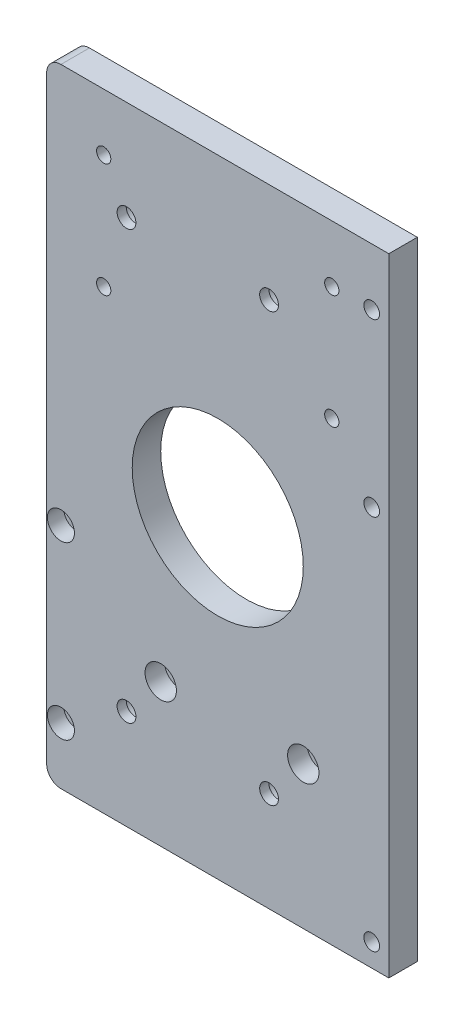
SolidWorks part; units mm, degrees
ref_plane "前视基准面" through (0, 0, 0) normal (0, 0, 1) x (1, 0, 0)
ref_plane "上视基准面" through (0, 0, 0) normal (0, 1, 0) x (1, 0, 0)
ref_plane "右视基准面" through (0, 0, 0) normal (1, 0, 0) x (0, 0, -1)
sketch "草图1" plane through (0, 0, 0) normal (0, 0, 1) x (1, 0, 0)
  line L1 (60, -110) -> (-60, -110)
  line L2 (60, -110) -> (60, 110)
  line L3 (60, 110) -> (-60, 110)
  line L4 (-60, -110) -> (-60, 110)
  line L5 (60, -110) -> (-60, 110) construction
  line L6 (60, 110) -> (-60, -110) construction
  point P0 (0, 0)
  dimension "D1" = 120
  dimension "D2" = 220
extrude "凸台-拉伸1" add sketch "草图1" along normal blind 10
hole_wizard "M6 螺纹孔1" positions "草图2" profile "草图3" tap size "M6" standard "GB" end condition up to next
sketch "草图2" plane through (0, 0, 0) normal (0, 0, -1) x (-1, 0, 0)
  line L0 (-40, 90) -> (40, 90) construction
  line L1 (40, 90) -> (40, 50) construction
  line L2 (40, 50) -> (-40, 50) construction
  line L3 (-40, 50) -> (-40, 90) construction
  line L6 (0, -110) -> (0, 50) construction
  line L7 (60, -110) -> (-60, -110) construction
  line L8 (-60, 110) -> (60, 110) construction
  point P0 (-40, 90)
  point P2 (-40, 50)
  point P4 (40, 90)
  point P6 (40, 50)
  dimension "D1" = 80
  dimension "D2" = 40
  dimension "D3" = 20
sketch "草图3" plane through (40, 90, 0) normal (1, 0, 0) x (0, 1, 0)
  line L0 (0, 0) -> (0, 10)
  line L1 (0, 10) -> (2.5, 10)
  line L2 (2.5, 10) -> (2.5, 0)
  line L5 (2.5, 0) -> (0, 0)
  line L11 (0, -6.35) -> (0, 107.95) construction
  dimension "通孔螺纹孔钻头直径" = 5
  dimension "通孔螺纹孔钻头深度" = 10
cosmetic thread "孔螺蚊线1" parameters "D2"=6
cosmetic thread "孔螺蚊线2" parameters "D2"=6
cosmetic thread "孔螺蚊线3" parameters "D2"=6
cosmetic thread "孔螺蚊线4" parameters "D2"=6
hole_wizard "打孔尺寸(%根据)内六角圆柱头螺钉的类型1" positions "草图4" profile "草图5" counterbore size "M6" standard "GB" end condition up to next
sketch "草图4" plane through (0, 0, 0) normal (0, 0, -1) x (-1, 0, 0)
  point P0 (32, -75)
  point P3 (-18, -75)
  point P6 (32, 75)
  point P9 (-18, 75)
sketch "草图5" plane through (-32, -75, 0) normal (1, 0, 0) x (0, 1, 0)
  line L0 (0, 0) -> (0, 10)
  line L1 (0, 10) -> (3.3, 10)
  line L3 (3.3, 10) -> (3.3, 6.8)
  line L4 (3.3, 6.8) -> (5.5, 6.8)
  line L5 (5.5, 6.8) -> (5.5, 0)
  line L7 (5.5, 0) -> (0, 0)
  line L11 (0, -6.35) -> (0, 107.95) construction
  dimension "通孔孔直径" = 6.6
  dimension "通孔孔深度" = 10
  dimension "柱形沉头孔直径" = 11
  dimension "柱形沉头孔深度" = 6.8
sketch "草图6" plane through (0, 0, 0) normal (0, 0, -1) x (-1, 0, 0)
  circle A2 centre (0, 0) radius 30
  dimension "D1" = 60
extrude "切除-拉伸1" cut sketch "草图6" against normal up to next
hole_wizard "打孔尺寸(%根据)内六角圆柱头螺钉的类型2" positions "草图7" profile "草图8" counterbore size "M5" standard "GB" end condition up to next
sketch "草图7" plane through (0, 0, 10) normal (0, 0, 1) x (1, 0, 0)
  point P0 (-55, -30)
  point P3 (-55, -90)
sketch "草图8" plane through (-55, -30, 10) normal (1, 0, 0) x (0, -1, 0)
  line L0 (0, 0) -> (0, 10)
  line L1 (0, 10) -> (2.75, 10)
  line L3 (2.75, 10) -> (2.75, 5.7)
  line L4 (2.75, 5.7) -> (4.75, 5.7)
  line L5 (4.75, 5.7) -> (4.75, 0)
  line L7 (4.75, 0) -> (0, 0)
  line L11 (0, -6.35) -> (0, 107.95) construction
  dimension "通孔孔直径" = 5.5
  dimension "通孔孔深度" = 10
  dimension "柱形沉头孔直径" = 9.5
  dimension "柱形沉头孔深度" = 5.7
hole_wizard "打孔尺寸(%根据)内六角圆柱头螺钉的类型3" positions "草图9" profile "草图10" counterbore size "M6" standard "GB" end condition up to next
sketch "草图9" plane through (0, 0, 10) normal (0, 0, 1) x (1, 0, 0)
  point P0 (-20, -60)
  point P3 (30, -60)
sketch "草图10" plane through (-20, -60, 10) normal (1, 0, 0) x (0, -1, 0)
  line L0 (0, 0) -> (0, 10)
  line L1 (0, 10) -> (3.3, 10)
  line L3 (3.3, 10) -> (3.3, 6.8)
  line L4 (3.3, 6.8) -> (5.5, 6.8)
  line L5 (5.5, 6.8) -> (5.5, 0)
  line L7 (5.5, 0) -> (0, 0)
  line L11 (0, -6.35) -> (0, 107.95) construction
  dimension "通孔孔直径" = 6.6
  dimension "通孔孔深度" = 10
  dimension "柱形沉头孔直径" = 11
  dimension "柱形沉头孔深度" = 6.8
hole_wizard "打孔尺寸(%根据)内六角圆柱头螺钉的类型4" positions "草图11" profile "草图12" counterbore size "M5" standard "GB" end condition up to next
sketch "草图11" plane through (0, 0, 0) normal (0, 0, -1) x (-1, 0, 0)
  point P0 (-54, 30)
  point P3 (-54, 90)
  point P6 (-54, -102)
sketch "草图12" plane through (54, 30, 0) normal (1, 0, 0) x (0, 1, 0)
  line L0 (0, 0) -> (0, 10)
  line L1 (0, 10) -> (2.75, 10)
  line L3 (2.75, 10) -> (2.75, 5.7)
  line L4 (2.75, 5.7) -> (5, 5.7)
  line L5 (5, 5.7) -> (5, 0)
  line L7 (5, 0) -> (0, 0)
  line L11 (0, -6.35) -> (0, 107.95) construction
  dimension "通孔孔直径" = 5.5
  dimension "通孔孔深度" = 10
  dimension "柱形沉头孔直径" = 10
  dimension "柱形沉头孔深度" = 5.7
fillet "圆角1" radius 5 2 edges at (-60, 110, 5) (-60, -110, 5)
